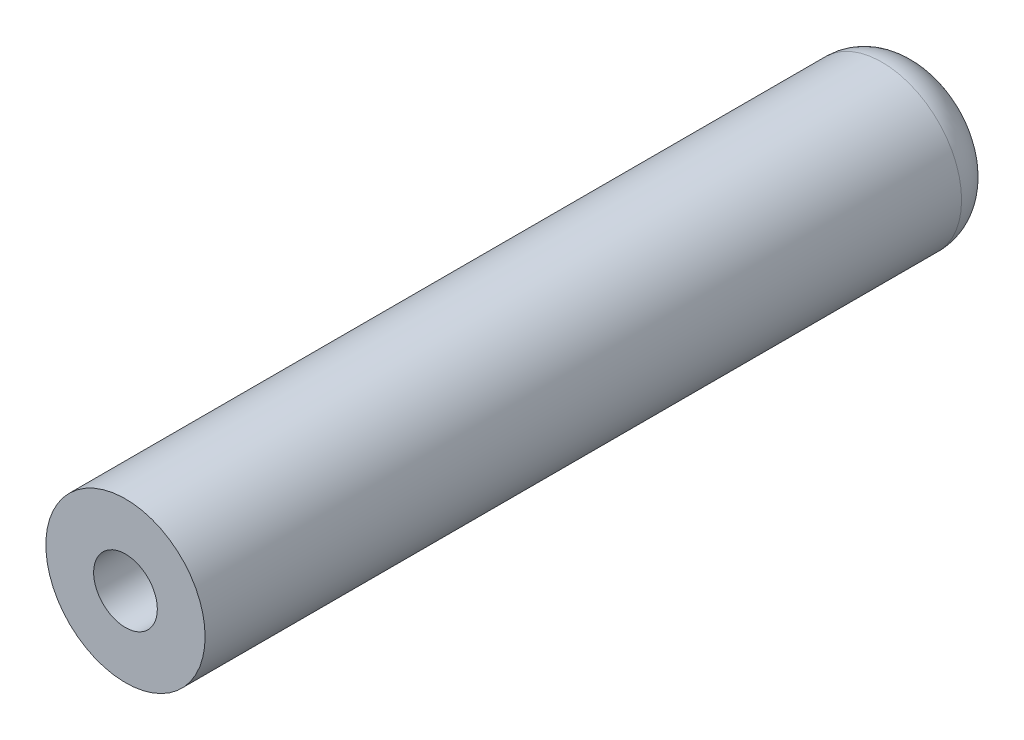
SolidWorks part; units mm, degrees
ref_plane "Front Plane" through (0, 0, 0) normal (0, 0, 1) x (1, 0, 0)
ref_plane "Top Plane" through (0, 0, 0) normal (0, 1, 0) x (1, 0, 0)
ref_plane "Right Plane" through (0, 0, 0) normal (1, 0, 0) x (0, 0, -1)
sketch "Sketch1" plane through (0, 0, 0) normal (0, 0, 1) x (1, 0, 0)
  circle A0 centre (10.2812, -38.2) radius 2
  dimension "D1" = 4
extrude "Boss-Extrude1" add sketch "Sketch1" along normal blind 20 contours A0
hole_wizard "M2 Tapped Hole1" positions "3DSketch2" profile "Sketch2" tap size "M2" standard "GB"
sketch3d "3DSketch2"
  line L0 (10.2812, -38.2, 20) -> (10.2812, -38.2, 23.7) construction
  point P0 (10.2812, -38.2, 23.7)
sketch "Sketch2" plane through (10.2812, -38.2, 23.7) normal (1, 0, 0) x (0, -1, 0)
  line L0 (0, 0) -> (0, 5.6807)
  line L1 (0, 5.6807) -> (0.8, 5.2)
  line L2 (0.8, 5.2) -> (0.8, 0)
  line L5 (0.8, 0) -> (0, 0)
  line L10 (0, 5.6807) -> (-0.8, 5.2) construction
  line L11 (0, -6.35) -> (0, 107.95) construction
  dimension "螺纹孔钻头直径" = 1.6
  dimension "螺纹孔钻头深度" = 5.2
  dimension "导头角度" = 118
cosmetic thread "Cosmetic thread1"
fillet "Fillet1" radius 1 1 edges at (12.2812, -38.2, 0)
